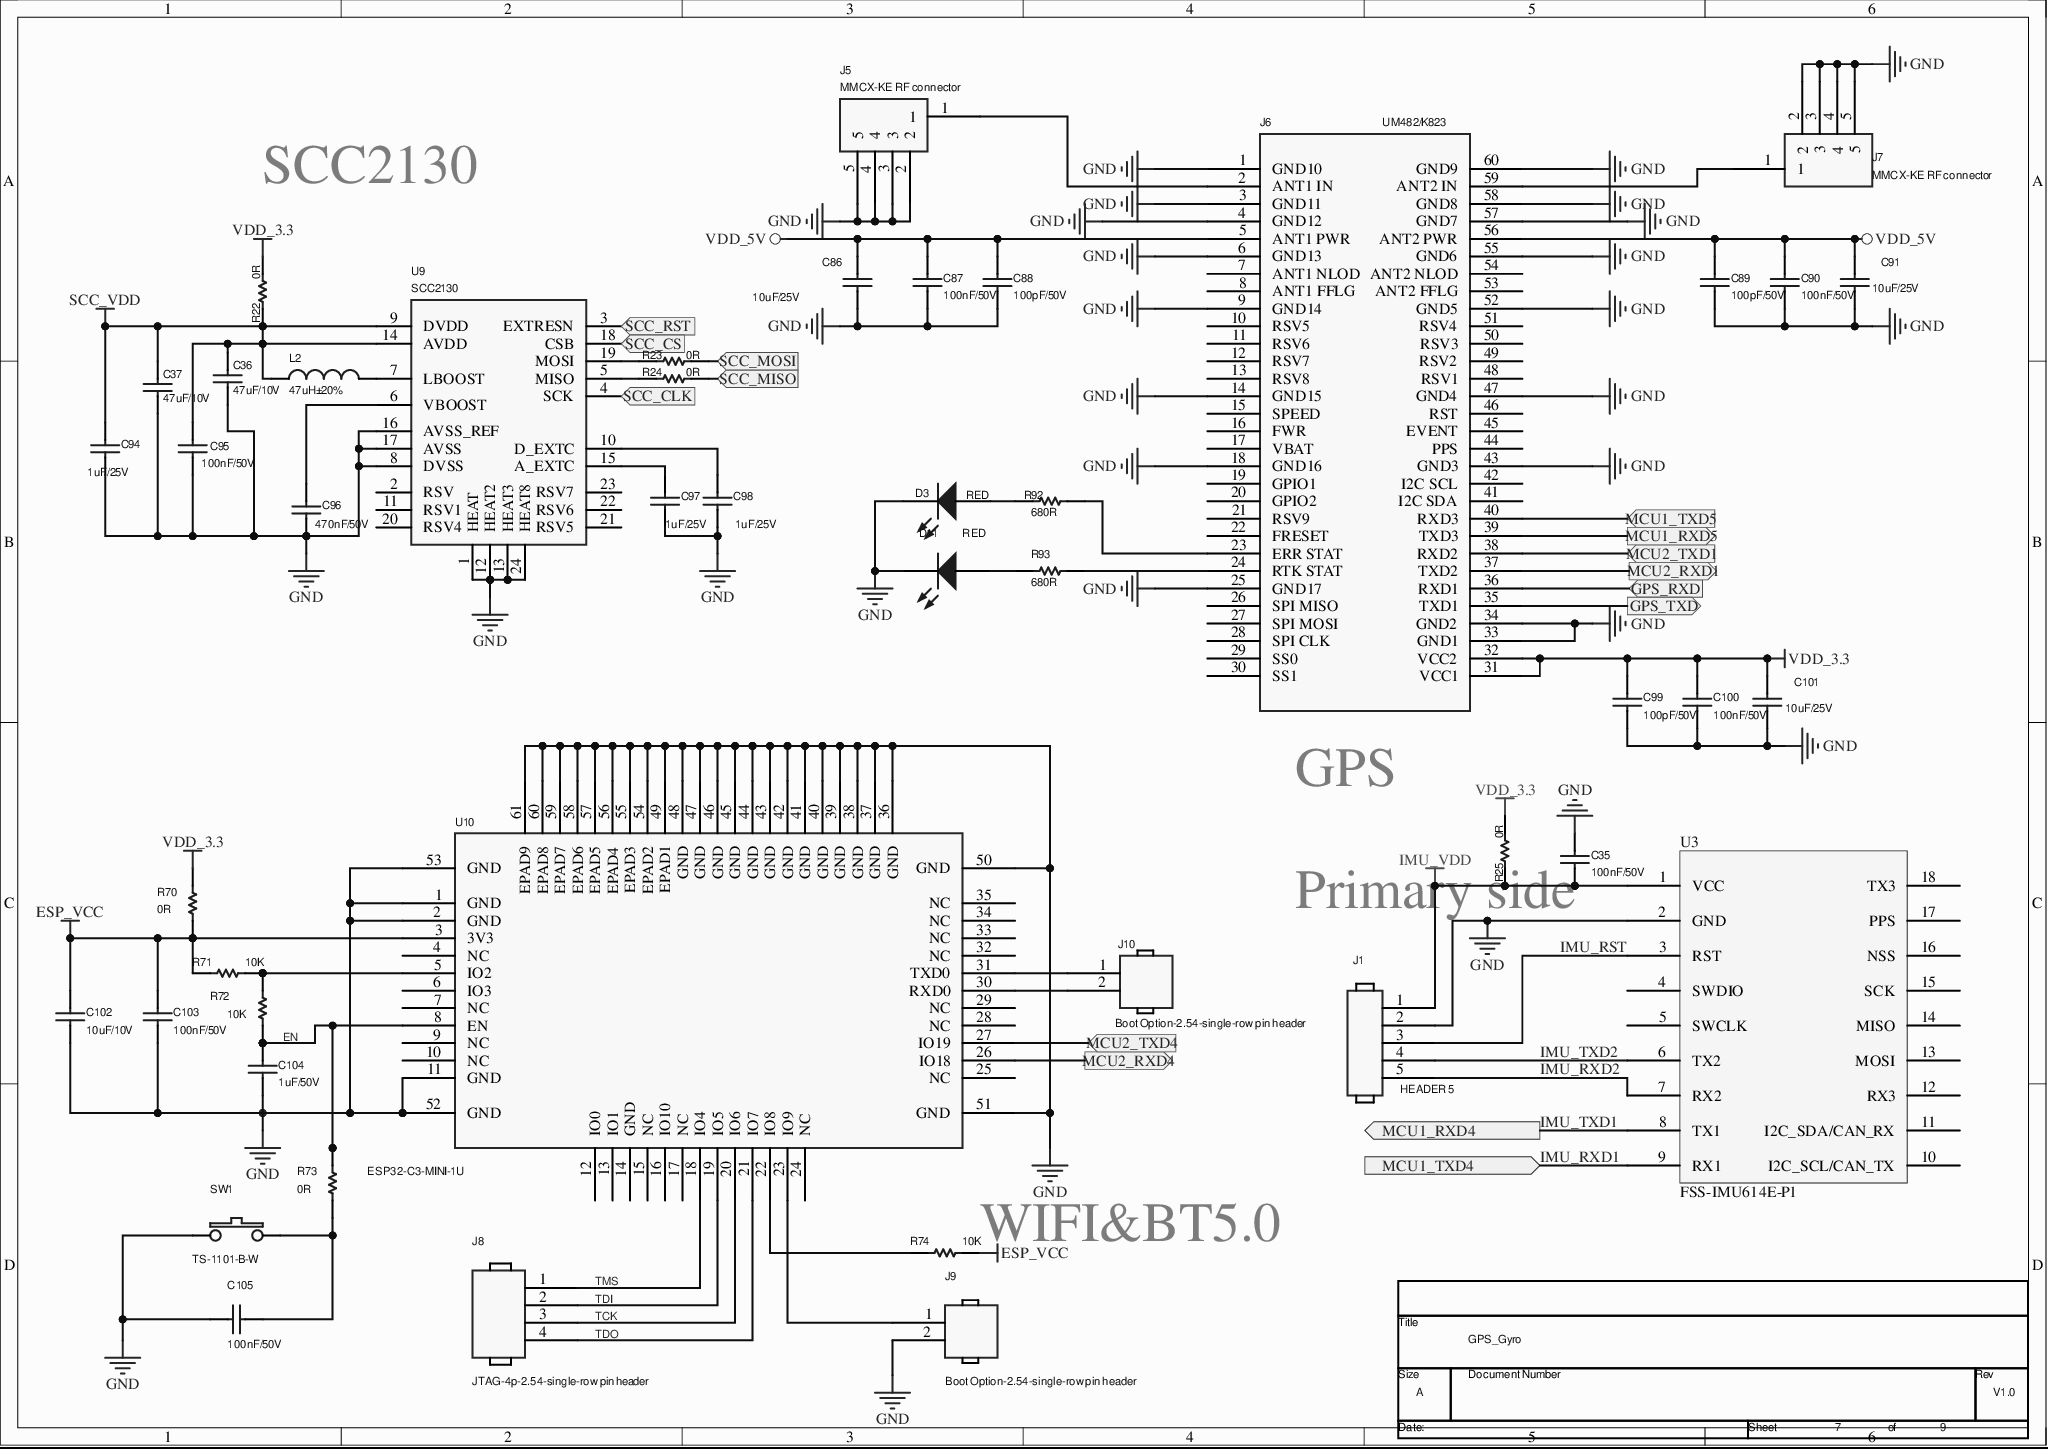
[diagram p0: MISC86294-14.SchDoc]
# Altium project MISC86294-22.PrjPcb (part 5 of 5)

## Sheet MISC86294-14.SchDoc
size 297 x 209 mm

### Parts
(Parts that share a designator on the sheet are numbered #1, #2 ... from top to bottom, then left to right.)
*#6  RevCode: V1.0  Title: GPS_Gyro  Page Size: A  Page Number: 7  Page Count: 9  (hidden comment: TitleBlock0)  (graphical)
C35  100nF/50V  [0603]
C36  47uF/10V  [CAP-SMD_L3.5-W2.8]
C37  47uF/10V  [CAP-SMD_L3.5-W2.8]
C86  10uF/25V  [C0805]
C87  100nF/50V  [0603]
C88  100pF/50V  [0603]
C89  100pF/50V  [0603]
C90  100nF/50V  [0603]
C91  10uF/25V  [C0805]
C94  1uF/25V  [0603]
C95  100nF/50V  [0603]
C96  470nF/50V  [0603]
C97  1uF/25V  [0603]
C98  1uF/25V  [0603]
C99  100pF/50V  [0603]
C100  100nF/50V  [0603]
C101  10uF/25V  [C0805]
C102  User_Value: 10uF/10V  [C0603]  (hidden comment: 100nF/50V)
C103  100nF/50V  [C0603]
C104  User_Value: 1uF/50V  [C0603]  (hidden comment: 100nF/50V)
C105  100nF/50V  [C0603]
D3  RED  [LED_0805]
D11  RED  [LED_0805]
J1  HEADER 5  [2.54mm_paizhen_5pin]
J5  MMCX-KE RF connector  [MMCX-KE]
J6  UM482/K823  [UM482_K823]
J7  MMCX-KE RF connector  [MMCX-KE]
J8  JTAG-4p-2.54-single-row pin header  [HDR_1X4_254]
J9  Boot Option-2.54-single-row pin header  [HDR_1X2_254]
J10  Boot Option-2.54-single-row pin header  [HDR_1X2_254]
L2  47uH±20%  [1210]
R22  0R  [R0603]
R23  0R  [R0603]
R24  0R  [R0603]
R25  0R  [R0603]
R70  0R  [R0603]
R71  10K  [R0603]
R72  10K  [R0603]
R73  0R  [R0603]
R74  10K  [R0603]
R92  User_Value: 680R  [0603]  (hidden comment: NA)
R93  User_Value: 680R  [0603]  (hidden comment: NA)
SW1  TS-1101-B-W  [SMD]
U3  FSS-IMU614E-P1  [FSS-IMU614E-P1]
U9  SCC2130  [SCC2130D]
U10  ESP32-C3-MINI-1U  [WIFIM-SMD_ESP32-C3-MINI-1]

### Ports
GPS_RXD (in), GPS_TXD (out), MCU1_RXD4 (out), MCU1_RXD5 (out), MCU1_TXD4 (in), MCU1_TXD5 (in), MCU2_RXD1 (out), MCU2_RXD4 (out), MCU2_TXD1 (in), MCU2_TXD4 (in), SCC_CLK (in), SCC_CS (in), SCC_MISO (in), SCC_MOSI (in), SCC_RST (in)

### Nets
ESP_VCC: C102.2 C103.2 R70.2 R71.2 R74.1 U10.3(3V3)
GND: C35.2 C36.2 C37.2 C86.1 C87.2 C88.2 C89.1 C90.1 C91.1 C94.2 C95.2 C96.2 C97.2 C98.2 C99.1 C100.1 C101.1 C102.1 C103.1 C104.1 C105.2 D3.2(K) D11.2(K) J1.2 J5.2 J5.3 J5.4 J5.5 J6.1(GND10) J6.3(GND11) J6.4(GND12) J6.6(GND13) J6.9(GND14) J6.14(GND15) J6.18(GND16) J6.25(GND17) J6.33(GND1) J6.34(GND2) J6.43(GND3) J6.47(GND4) J6.52(GND5) J6.55(GND6) J6.57(GND7) J6.58(GND8) J6.60(GND9) J7.2 J7.3 J7.4 J7.5 J9.2 SW1.1 U3.2(GND) U9.1(HEAT) U9.8(DVSS) U9.12(HEAT2) U9.13(HEAT3) U9.16(AVSS_REF) U9.17(AVSS) U9.24(HEAT8) U10.1(GND) U10.2(GND) U10.11(GND) U10.36(GND) U10.37(GND) U10.38(GND) U10.39(GND) U10.40(GND) U10.41(GND) U10.42(GND) U10.43(GND) U10.44(GND) U10.45(GND) U10.46(GND) U10.47(GND) U10.48(GND) U10.49(EPAD1) U10.50(GND) U10.51(GND) U10.52(GND) U10.53(GND) U10.54(EPAD2) U10.55(EPAD3) U10.56(EPAD4) U10.57(EPAD5) U10.58(EPAD6) U10.59(EPAD7) U10.60(EPAD8) U10.61(EPAD9)
IMU_VDD: C35.1 J1.1 R25.2 U3.1(VCC)
SCC_VDD: C36.1 C37.1 C94.1 C95.1 L2.1 R22.2 U9.9(DVDD) U9.14(AVDD)
VDD_3.3: C99.2 C100.2 C101.2 J6.31(VCC1) J6.32(VCC2) R22.1 R25.1 R70.1
VDD_5V: C86.2 C87.1 C88.1 C89.2 C90.2 C91.2 J6.5(ANT1_PWR) J6.56(ANT2_PWR)
EN: C104.2 R72.2 R73.1 U10.8(EN)
IMU_RST: J1.3 U3.3(RST)
IMU_RXD1: U3.9(RX1) ; port MCU1_TXD4
IMU_RXD2: J1.5 U3.7(RX2)
IMU_TXD1: U3.8(TX1) ; port MCU1_RXD4
IMU_TXD2: J1.4 U3.6(TX2)
TCK: J8.3 U10.20(IO6)
TDI: J8.2 U10.19(IO5)
TDO: J8.4 U10.21(IO7)
TMS: J8.1 U10.18(IO4)
NetC96_1: C96.1 U9.6(VBOOST)
NetC97_1: C97.1 U9.15(A_EXTC)
NetC98_1: C98.1 U9.10(D_EXTC)
NetC105_1: C105.1 R73.2 SW1.2
NetD3_1: D3.1(A) R92.2
NetD11_1: D11.1(A) R93.2
NetJ5_1: J5.1 J6.2(ANT1_IN)
NetJ6_23: J6.23(ERR_STAT) R92.1
NetJ6_24: J6.24(RTK_STAT) R93.1
NetJ6_35: J6.35(TXD1) ; port GPS_TXD
NetJ6_36: J6.36(RXD1) ; port GPS_RXD
NetJ6_37: J6.37(TXD2) ; port MCU2_RXD1
NetJ6_38: J6.38(RXD2) ; port MCU2_TXD1
NetJ6_39: J6.39(TXD3) ; port MCU1_RXD5
NetJ6_40: J6.40(RXD3) ; port MCU1_TXD5
NetJ6_59: J6.59(ANT2_IN) J7.1
NetJ9_1: J9.1 U10.23(IO9)
NetJ10_1: J10.1 U10.31(TXD0)
NetJ10_2: J10.2 U10.30(RXD0)
NetJ19_1: U10.27(IO19) ; port MCU2_TXD4
NetJ19_2: U10.26(IO18) ; port MCU2_RXD4
NetL2_2: L2.2 U9.7(LBOOST)
NetR23_1: R23.1 ; port SCC_MOSI
NetR23_2: R23.2 U9.19(MOSI)
NetR24_1: R24.1 ; port SCC_MISO
NetR24_2: R24.2 U9.5(MISO)
NetR71_1: R71.1 R72.1 U10.5(IO2)
NetR74_2: R74.2 U10.22(IO8)
NetU1_40: U9.18(CSB) ; port SCC_CS
NetU1_41: U9.4(SCK) ; port SCC_CLK
NetU1_44: U9.3(EXTRESN) ; port SCC_RST

Not connected (* = marked no-connect by the designer): J6 7(ANT1_NLOD) 8(ANT1_FFLG) 10(RSV5) 11(RSV6) 12(RSV7) 13(RSV8) 15(SPEED) 16(FWR) 17(VBAT) 19(GPIO1) 20(GPIO2) 21(RSV9) 22(FRESET) 26(SPI_MISO) 27(SPI_MOSI) 28(SPI_CLK) 29(SS0) 30(SS1) 41(I2C_SDA) 42(I2C_SCL) 44(PPS) 45(EVENT) 46(RST) 48(RSV1) 49(RSV2) 50(RSV3) 51(RSV4) 53(ANT2_FFLG) 54(ANT2_NLOD); U3 4(SWDIO) 5(SWCLK) 10(I2C_SCL/CAN_TX) 11(I2C_SDA/CAN_RX) 12(RX3) 13(MOSI) 14(MISO) 15(SCK) 16(NSS) 17(PPS) 18(TX3); U9 2(RSV) 11(RSV1) 20(RSV4) 21(RSV5) 22(RSV6) 23(RSV7); U10 4(NC) 6(IO3) 7(NC) 9(NC) 10(NC) 12(IO0) 13(IO1) 14(GND) 15(NC) 16(IO10) 17(NC) 24(NC) 25(NC) 28(NC) 29(NC) 32(NC) 33(NC) 34(NC) 35(NC)

### Notes on the sheet
- SCC2130
- (near J6) GPS
- Primary side
- (near R74) WIFI&BT5.0

### Library data of the parts
*#6 = TitleBlock0: Document: Agr-Ctrl-3GS-07; Page Create Date: March  8, 1995
C35 C100 = Cap_C17: Kind: General; SubKind: Capacitor; Origin: Altium; Published: 8-Jun-2000; LatestRevisionDate: 17-Jul-2002; LatestRevisionNote: Re-released for DXP Platform.; PackageReference: RAD-0.3; User_Value: 100nF/50V; Created: 1/08/1993; Spice Prefix: C; Type: Capacitor; Publisher: Altium Limited
C36 C37 = Cap_C2: Origin: Altium; Published: 8-Jun-2000; LatestRevisionDate: 17-Jul-2002; LatestRevisionNote: Re-released for DXP Platform.; PackageReference: RAD-0.3; User_Value: 47uF/10V; Created: 1/08/1993; Publisher: Altium Limited
C86 = Cap_C3: Kind: General; SubKind: Capacitor; Origin: Altium; Published: 8-Jun-2000; LatestRevisionDate: 17-Jul-2002; LatestRevisionNote: Re-released for DXP Platform.; PackageReference: RAD-0.3; User_Value: 10uF/25V; Created: 1/08/1993; Spice Prefix: C; Type: Capacitor; Publisher: Altium Limited
C87 = Cap_C5: Kind: General; SubKind: Capacitor; Origin: Altium; Published: 8-Jun-2000; LatestRevisionDate: 17-Jul-2002; LatestRevisionNote: Re-released for DXP Platform.; PackageReference: RAD-0.3; User_Value: 100nF/50V; Created: 1/08/1993; Spice Prefix: C; Type: Capacitor; Publisher: Altium Limited
C88 = Cap_C6: Kind: General; SubKind: Capacitor; Origin: Altium; Published: 8-Jun-2000; LatestRevisionDate: 17-Jul-2002; LatestRevisionNote: Re-released for DXP Platform.; PackageReference: RAD-0.3; User_Value: 100pF/50V; Created: 1/08/1993; Spice Prefix: C; Type: Capacitor; Publisher: Altium Limited
C89 = Cap_C7: Kind: General; SubKind: Capacitor; Origin: Altium; Published: 8-Jun-2000; LatestRevisionDate: 17-Jul-2002; LatestRevisionNote: Re-released for DXP Platform.; PackageReference: RAD-0.3; User_Value: 100pF/50V; Created: 1/08/1993; Spice Prefix: C; Type: Capacitor; Publisher: Altium Limited
C90 = Cap_C8: Kind: General; SubKind: Capacitor; Origin: Altium; Published: 8-Jun-2000; LatestRevisionDate: 17-Jul-2002; LatestRevisionNote: Re-released for DXP Platform.; PackageReference: RAD-0.3; User_Value: 100nF/50V; Created: 1/08/1993; Spice Prefix: C; Type: Capacitor; Publisher: Altium Limited
C91 = Cap_C4: Kind: General; SubKind: Capacitor; Origin: Altium; Published: 8-Jun-2000; LatestRevisionDate: 17-Jul-2002; LatestRevisionNote: Re-released for DXP Platform.; PackageReference: RAD-0.3; User_Value: 10uF/25V; Created: 1/08/1993; Spice Prefix: C; Type: Capacitor; Publisher: Altium Limited
C94 = Cap_C9: Kind: General; SubKind: Capacitor; Origin: Altium; Published: 8-Jun-2000; Revision: July-2002: Re-released for DXP Platform.; User_Value: 1uF/25V; Spice Prefix: C; Type: Capacitor; Publisher: Altium Limited
C95 = Cap_C10: Kind: General; SubKind: Capacitor; Origin: Altium; Published: 8-Jun-2000; Revision: July-2002: Re-released for DXP Platform.; User_Value: 100nF/50V; Spice Prefix: C; Type: Capacitor; Publisher: Altium Limited
C96 = Cap_C13: Kind: General; SubKind: Capacitor; Origin: Altium; Published: 8-Jun-2000; Revision: July-2002: Re-released for DXP Platform.; User_Value: 470nF/50V; Spice Prefix: C; Type: Capacitor; Publisher: Altium Limited
C97 = Cap_C11: Kind: General; SubKind: Capacitor; Origin: Altium; Published: 8-Jun-2000; Revision: July-2002: Re-released for DXP Platform.; User_Value: 1uF/25V; Spice Prefix: C; Type: Capacitor; Publisher: Altium Limited
C98 = Cap_C12: Kind: General; SubKind: Capacitor; Origin: Altium; Published: 8-Jun-2000; Revision: July-2002: Re-released for DXP Platform.; User_Value: 1uF/25V; Spice Prefix: C; Type: Capacitor; Publisher: Altium Limited
C99 = Cap_C16: Kind: General; SubKind: Capacitor; Origin: Altium; Published: 8-Jun-2000; LatestRevisionDate: 17-Jul-2002; LatestRevisionNote: Re-released for DXP Platform.; PackageReference: RAD-0.3; User_Value: 100pF/50V; Created: 1/08/1993; Spice Prefix: C; Type: Capacitor; Publisher: Altium Limited
C101 = Cap_C15: Kind: General; SubKind: Capacitor; Origin: Altium; Published: 8-Jun-2000; LatestRevisionDate: 17-Jul-2002; LatestRevisionNote: Re-released for DXP Platform.; PackageReference: RAD-0.3; User_Value: 10uF/25V; Created: 1/08/1993; Spice Prefix: C; Type: Capacitor; Publisher: Altium Limited
C102-C105 = Cap_C90: Kind: General; SubKind: Capacitor; Origin: Altium; Published: 8-Jun-2000; LatestRevisionDate: 17-Jul-2002; LatestRevisionNote: Re-released for DXP Platform.; PackageReference: RAD-0.3; Created: 1/08/1993; Spice Prefix: C; Type: Capacitor; Publisher: Altium Limited
  C103 C105: User_Value: 100nF/50V
D3 D11 = LED1_D4: Kind: General; SubKind: Diode; Origin: Altium; Published: 8-Jun-2000; LatestRevisionDate: 08-Jul-2005; LatestRevisionNote: Mech Layer 1 removed.; PackageReference: LED-1; Spice Prefix: D; Publisher: Altium Limited
J5 = CIRCLE_J1: Origin: Altium
J6 = UM482_J2: Origin: Altium
J7 = CIRCLE_J3: Origin: Altium
J8 = HEADER 4
J9 J10 = HEADER 2
L2 = Inductor_L1: Code_IEC: 1005; Origin: Altium; Published: 8-Jun-2000; LatestRevisionDate: 29-May-2009; LatestRevisionNote: IPC-7351 Footprint Added.; PackageReference: 0402-A; PackageDescription: Chip Inductor; Code_JEITA: 0402; User_Value: 47uH±20%; Created: 28/07/2004; Publisher: Altium Limited
R22-R25 R70-R74 = Res1_R57: Kind: General; SubKind: Resistor; Origin: Altium; Published: 8-Jun-2000; LatestRevisionDate: 17-Jul-2002; LatestRevisionNote: Re-released for DXP Platform.; PackageReference: AXIAL-0.3; Created: 1/08/1993; Spice Prefix: R; Type: Resistor; Publisher: Altium Limited
  R22-R25 R70 R73: User_Value: 0R
  R71 R72 R74: User_Value: 10K
R92 R93 = Res1_R8: Origin: Altium; Published: 8-Jun-2000; LatestRevisionDate: 17-Jul-2002; LatestRevisionNote: Re-released for DXP Platform.; PackageReference: AXIAL-0.3; Publisher: Altium Limited
SW1 = SW_PB_SPST
U3 = FSS-IMU614-AG
U9 = SCC2130_U2: Origin: Altium

## Sheet MISC86294-16.SchDoc
size 297 x 209 mm
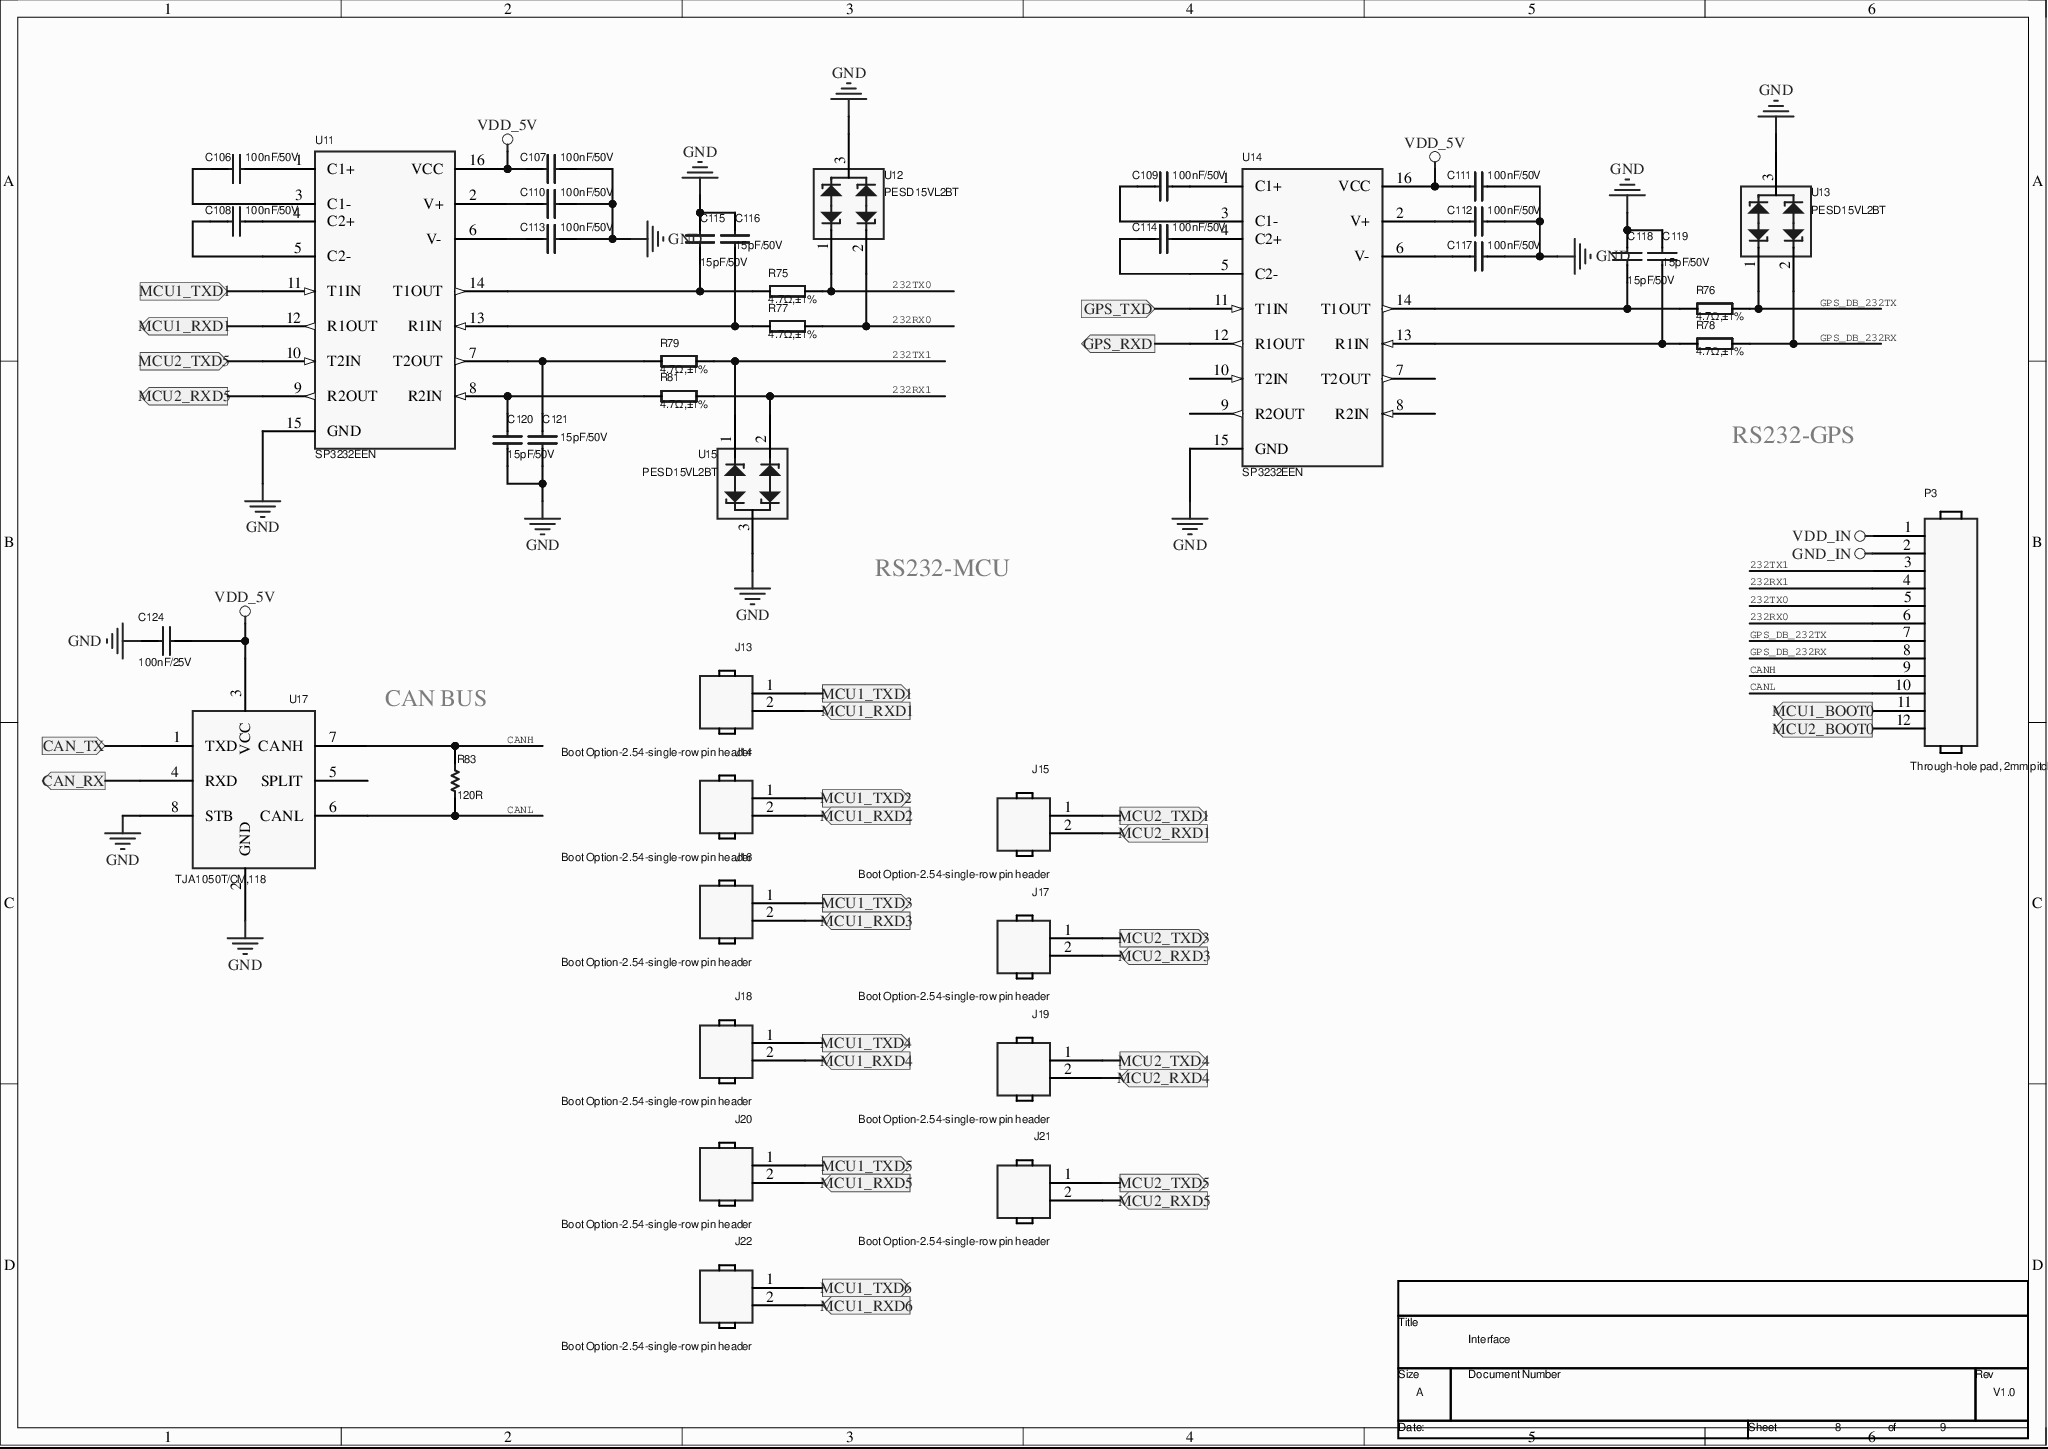
[diagram p1: MISC86294-16.SchDoc]

### Parts
(Parts that share a designator on the sheet are numbered #1, #2 ... from top to bottom, then left to right.)
*#7  RevCode: V1.0  Title: Interface  Page Size: A  Page Number: 8  Page Count: 9  (hidden comment: TitleBlock0)  (graphical)
C106  100nF/50V  [0603]
C107  100nF/50V  [0603]
C108  100nF/50V  [0603]
C109  100nF/50V  [0603]
C110  100nF/50V  [0603]
C111  100nF/50V  [0603]
C112  100nF/50V  [0603]
C113  100nF/50V  [0603]
C114  100nF/50V  [0603]
C115  15pF/50V  [0603]
C116  15pF/50V  [0603]
C117  100nF/50V  [0603]
C118  15pF/50V  [0603]
C119  15pF/50V  [0603]
C120  15pF/50V  [0603]
C121  15pF/50V  [0603]
C124  User_Value: 100nF/25V  [C0603]  (hidden comment: 100nF/50V)
J13  Boot Option-2.54-single-row pin header  [HDR_1X2_254]
J14  Boot Option-2.54-single-row pin header  [HDR_1X2_254]
J15  Boot Option-2.54-single-row pin header  [HDR_1X2_254]
J16  Boot Option-2.54-single-row pin header  [HDR_1X2_254]
J17  Boot Option-2.54-single-row pin header  [HDR_1X2_254]
J18  Boot Option-2.54-single-row pin header  [HDR_1X2_254]
J19  Boot Option-2.54-single-row pin header  [HDR_1X2_254]
J20  Boot Option-2.54-single-row pin header  [HDR_1X2_254]
J21  Boot Option-2.54-single-row pin header  [HDR_1X2_254]
J22  Boot Option-2.54-single-row pin header  [HDR_1X2_254]
P3  Through-hole pad, 2mm pitch  [XH-12A]
R75  4.7Ω,±1%  [0603]
R76  4.7Ω,±1%  [0603]
R77  4.7Ω,±1%  [0603]
R78  4.7Ω,±1%  [0603]
R79  4.7Ω,±1%  [0603]
R81  4.7Ω,±1%  [0603]
R83  120R  [R0603]
U11  SP3232EEN  [SOP16-6_6]
U12  PESD15VL2BT  [SOT-23]
U13  PESD15VL2BT  [SOT-23]
U14  SP3232EEN  [SOP16-6_6]
U15  PESD15VL2BT  [SOT-23]
U17  TJA1050T/CM,118  [SOIC-8]

### Ports
CAN_RX (out), CAN_TX (in), GPS_RXD (out), GPS_TXD (in), MCU1_BOOT0 (out), MCU1_RXD1 (in), MCU1_RXD1 (out), MCU1_RXD2 (in), MCU1_RXD3 (in), MCU1_RXD4 (in), MCU1_RXD5 (in), MCU1_RXD6 (in), MCU1_TXD1 (in), MCU1_TXD1 (out), MCU1_TXD2 (out), MCU1_TXD3 (out), MCU1_TXD4 (out), MCU1_TXD5 (out), MCU1_TXD6 (out), MCU2_BOOT0 (out), MCU2_RXD1 (in), MCU2_RXD3 (in), MCU2_RXD4 (in), MCU2_RXD5 (in), MCU2_RXD5 (out), MCU2_TXD1 (out), MCU2_TXD3 (out), MCU2_TXD4 (out), MCU2_TXD5 (in), MCU2_TXD5 (out)

### Nets
GND: C107.2 C110.2 C111.2 C112.2 C113.2 C115.1 C116.1 C117.2 C118.1 C119.1 C120.2 C121.2 C124.1 U11.15(GND) U12.3 U13.3 U14.15(GND) U15.3 U17.2(GND) U17.8(STB)
GND_IN: P3.2
VDD_5V: C107.1 C111.1 C124.2 U11.16(VCC) U14.16(VCC) U17.3(VCC)
VDD_IN: P3.1
232RX0: P3.6 R77.1 U12.2
232RX1: P3.4 R81.1 U15.2
232TX0: P3.5 R75.1 U12.1
232TX1: P3.3 R79.1 U15.1
CANH: P3.9 R83.1 U17.7(CANH)
CANL: P3.10 R83.2 U17.6(CANL)
GPS_DB_232RX: P3.8 R78.1 U13.2
GPS_DB_232TX: P3.7 R76.1 U13.1
IMU_RXD1: J18.1 ; port MCU1_TXD4
IMU_TXD1: J18.2 ; port MCU1_RXD4
NetC106_1: C106.1 U11.3(C1-)
NetC106_2: C106.2 U11.1(C1+)
NetC108_1: C108.1 U11.5(C2-)
NetC108_2: C108.2 U11.4(C2+)
NetC109_1: C109.1 U14.3(C1-)
NetC109_2: C109.2 U14.1(C1+)
NetC110_1: C110.1 U11.2(V+)
NetC112_1: C112.1 U14.2(V+)
NetC113_1: C113.1 U11.6(V-)
NetC114_1: C114.1 U14.5(C2-)
NetC114_2: C114.2 U14.4(C2+)
NetC115_2: C115.2 R75.2 U11.14(T1OUT)
NetC116_2: C116.2 R77.2 U11.13(R1IN)
NetC117_1: C117.1 U14.6(V-)
NetC118_2: C118.2 R76.2 U14.14(T1OUT)
NetC119_2: C119.2 R78.2 U14.13(R1IN)
NetC120_1: C120.1 R81.2 U11.8(R2IN)
NetC121_1: C121.1 R79.2 U11.7(T2OUT)
NetJ6_35: U14.11(T1IN) ; port GPS_TXD
NetJ6_36: U14.12(R1OUT) ; port GPS_RXD
NetJ6_37: J15.2 ; port MCU2_RXD1
NetJ6_38: J15.1 ; port MCU2_TXD1
NetJ6_39: J20.2 ; port MCU1_RXD5
NetJ6_40: J20.1 ; port MCU1_TXD5
NetJ13_1: J13.1 U11.11(T1IN) ; port MCU1_TXD1
NetJ13_2: J13.2 U11.12(R1OUT) ; port MCU1_RXD1
NetJ14_1: J14.1 ; port MCU1_TXD2
NetJ14_2: J14.2 ; port MCU1_RXD2
NetJ16_1: J16.1 ; port MCU1_TXD3
NetJ16_2: J16.2 ; port MCU1_RXD3
NetJ17_1: J17.1 ; port MCU2_TXD3
NetJ17_2: J17.2 ; port MCU2_RXD3
NetJ19_1: J19.1 ; port MCU2_TXD4
NetJ19_2: J19.2 ; port MCU2_RXD4
NetJ21_1: J21.1 U11.10(T2IN) ; port MCU2_TXD5
NetJ21_2: J21.2 U11.9(R2OUT) ; port MCU2_RXD5
NetJ22_1: J22.1 ; port MCU1_TXD6
NetJ22_2: J22.2 ; port MCU1_RXD6
NetP3_11: P3.11 ; port MCU1_BOOT0
NetP3_12: P3.12 ; port MCU2_BOOT0
NetU1_103: U17.4(RXD) ; port CAN_RX
NetU1_104: U17.1(TXD) ; port CAN_TX

Not connected (* = marked no-connect by the designer): U14 7(T2OUT) 8(R2IN) 9(R2OUT) 10(T2IN); U17 5(SPLIT)

### Notes on the sheet
- RS232-GPS
- RS232-MCU
- CAN BUS

### Library data of the parts
*#7 = TitleBlock0: Document: Agr-Ctrl-3GS-08; Page Create Date: March  8, 1995
C106 = Cap_C18: Origin: Altium; Published: 8-Jun-2000; Revision: July-2002: Re-released for DXP Platform.; User_Value: 100nF/50V; Publisher: Altium Limited
C107 = Cap_C19: Origin: Altium; Published: 8-Jun-2000; Revision: July-2002: Re-released for DXP Platform.; User_Value: 100nF/50V; Publisher: Altium Limited
C108 = Cap_C21: Origin: Altium; Published: 8-Jun-2000; Revision: July-2002: Re-released for DXP Platform.; User_Value: 100nF/50V; Publisher: Altium Limited
C109 = Cap_C36: Origin: Altium; Published: 8-Jun-2000; Revision: July-2002: Re-released for DXP Platform.; User_Value: 100nF/50V; Publisher: Altium Limited
C110 = Cap_C20: Origin: Altium; Published: 8-Jun-2000; Revision: July-2002: Re-released for DXP Platform.; User_Value: 100nF/50V; Publisher: Altium Limited
C111 = Cap_C37: Origin: Altium; Published: 8-Jun-2000; Revision: July-2002: Re-released for DXP Platform.; User_Value: 100nF/50V; Publisher: Altium Limited
C112 = Cap_C38: Origin: Altium; Published: 8-Jun-2000; Revision: July-2002: Re-released for DXP Platform.; User_Value: 100nF/50V; Publisher: Altium Limited
C113 = Cap_C24: Origin: Altium; Published: 8-Jun-2000; Revision: July-2002: Re-released for DXP Platform.; User_Value: 100nF/50V; Publisher: Altium Limited
C114 = Cap_C39: Origin: Altium; Published: 8-Jun-2000; Revision: July-2002: Re-released for DXP Platform.; User_Value: 100nF/50V; Publisher: Altium Limited
C115 = Cap_C22: Origin: Altium; Published: 8-Jun-2000; Revision: July-2002: Re-released for DXP Platform.; User_Value: 15pF/50V; Publisher: Altium Limited
C116 = Cap_C23: Origin: Altium; Published: 8-Jun-2000; Revision: July-2002: Re-released for DXP Platform.; User_Value: 15pF/50V; Publisher: Altium Limited
C117 = Cap_C42: Origin: Altium; Published: 8-Jun-2000; Revision: July-2002: Re-released for DXP Platform.; User_Value: 100nF/50V; Publisher: Altium Limited
C118 = Cap_C40: Origin: Altium; Published: 8-Jun-2000; Revision: July-2002: Re-released for DXP Platform.; User_Value: 15pF/50V; Publisher: Altium Limited
C119 = Cap_C41: Origin: Altium; Published: 8-Jun-2000; Revision: July-2002: Re-released for DXP Platform.; User_Value: 15pF/50V; Publisher: Altium Limited
C120 = Cap_C26: Origin: Altium; Published: 8-Jun-2000; Revision: July-2002: Re-released for DXP Platform.; User_Value: 15pF/50V; Publisher: Altium Limited
C121 = Cap_C27: Origin: Altium; Published: 8-Jun-2000; Revision: July-2002: Re-released for DXP Platform.; User_Value: 15pF/50V; Publisher: Altium Limited
C124 = Cap_C106: Kind: General; SubKind: Capacitor; Origin: Altium; Published: 8-Jun-2000; LatestRevisionDate: 17-Jul-2002; LatestRevisionNote: Re-released for DXP Platform.; PackageReference: RAD-0.3; Created: 1/08/1993; Spice Prefix: C; Type: Capacitor; Publisher: Altium Limited
J13-J22 = HEADER 2
P3 = HEADER 12
R75 = RES_R14: Origin: Altium; User_Value: 4.7Ω,±1%
R76 = RES_R22: Origin: Altium; User_Value: 4.7Ω,±1%
R77 = RES_R16: Origin: Altium; User_Value: 4.7Ω,±1%
R78 = RES_R23: Origin: Altium; User_Value: 4.7Ω,±1%
R79 = RES_R17: Origin: Altium; User_Value: 4.7Ω,±1%
R81 = RES_R18: Origin: Altium; User_Value: 4.7Ω,±1%
R83 = Res1_R90: Kind: General; SubKind: Resistor; Origin: Altium; Published: 8-Jun-2000; LatestRevisionDate: 17-Jul-2002; LatestRevisionNote: Re-released for DXP Platform.; PackageReference: AXIAL-0.3; User_Value: 120R; Created: 1/08/1993; Spice Prefix: R; Type: Resistor; Publisher: Altium Limited
U11 = SP202ECT_U3: Origin: Altium
U12 = PESD12VL2BT_U4: Origin: Altium
U13 = PESD12VL2BT_U8: Origin: Altium
U14 = SP202ECT_U7: Origin: Altium
U15 = PESD12VL2BT_U5: Origin: Altium
U17 = TJA1040T_U18: Origin: Altium

## Sheet MISC86294-18.SchDoc
size 297 x 209 mm
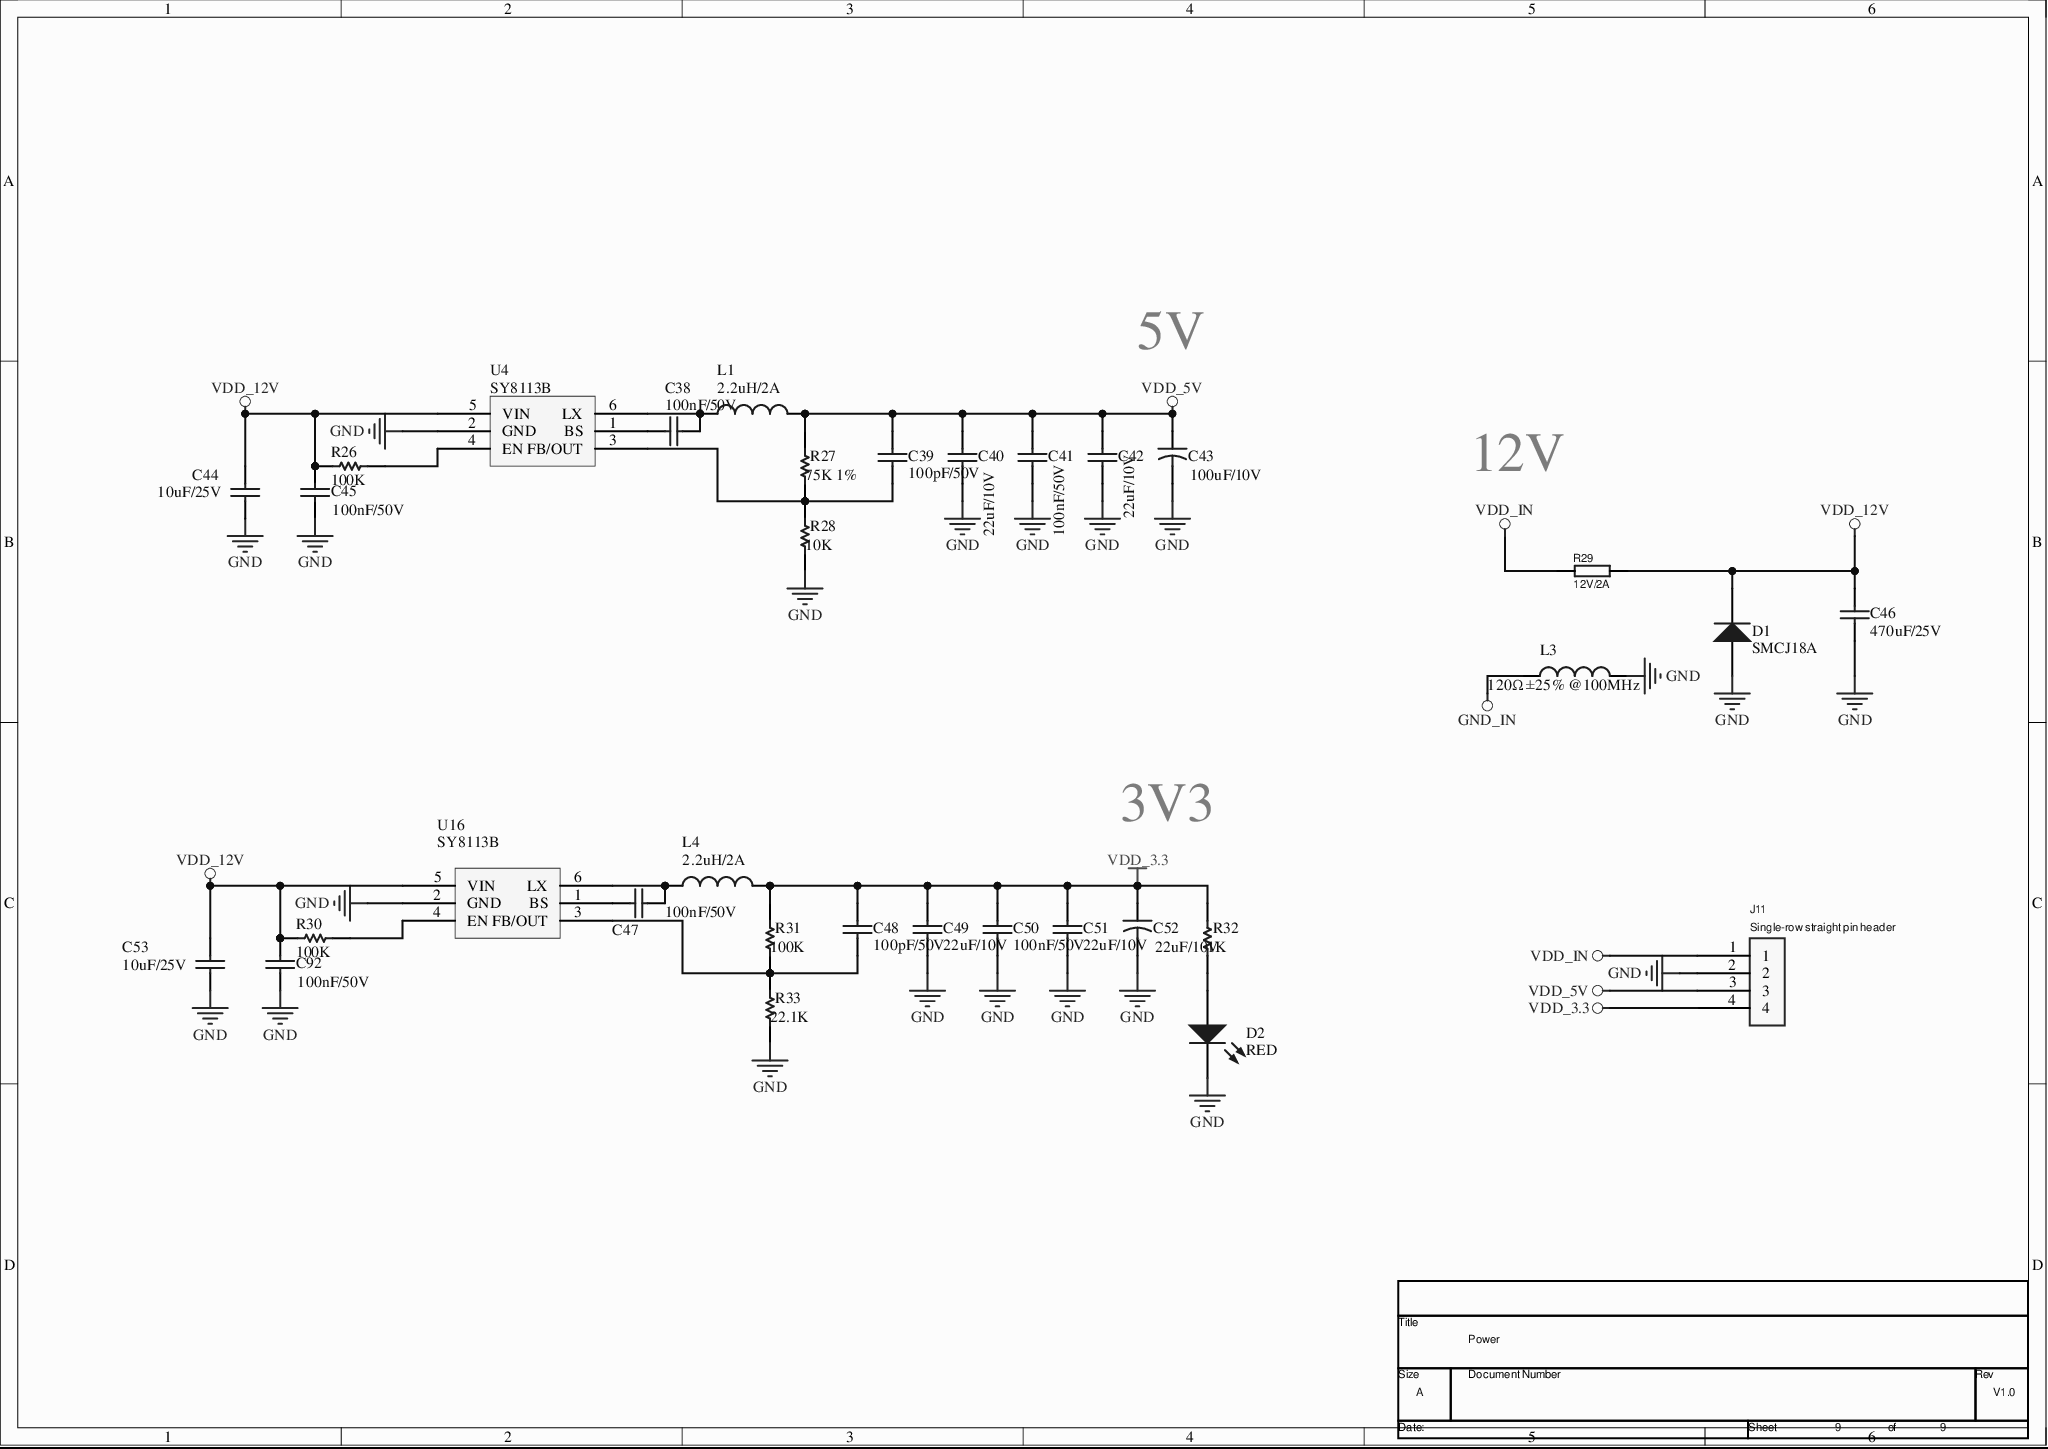
[diagram p2: MISC86294-18.SchDoc]

### Parts
(Parts that share a designator on the sheet are numbered #1, #2 ... from top to bottom, then left to right.)
*#8  RevCode: V1.0  Title: Power  Page Size: A  Page Number: 9  (hidden comment: TitleBlock0)  (graphical)
C38  100nF/50V  [0603]
C39  100pF/50V  [0603]
C40  22uF/10V  [C0805]
C41  100nF/50V  [0603]
C42  22uF/10V  [C0805]
C43  100uF/10V  [CAP-TH_BD5.0-P2.00-D0.8-FD]
C44  10uF/25V  [C0805]
C45  100nF/50V  [0603]
C46  470uF/25V  [CAP-TH_BD8.0-P3.50-D1.0-FD]
C47  100nF/50V  [0603]
C48  100pF/50V  [0603]
C49  22uF/10V  [C0805]
C50  100nF/50V  [0603]
C51  22uF/10V  [C0805]
C52  22uF/10V  [C0805]
C53  10uF/25V  [C0805]
C92  100nF/50V  [0603]
D1  SMCJ18A  [SMC_L6.9-W5.9-LS7.9-RD]
D2  RED  [LED_0805]
J11  Single-row straight pin header  [HDR1X4]
L1  2.2uH/2A  [IND-SMD_L4.0-W4.0]
L3  120Ω ±25% @100MHz  [0603]
L4  2.2uH/2A  [IND-SMD_L4.0-W4.0]
R26  100K  [0603]
R27  75K 1%  [0603]
R28  10K  [0603]
R29  12V/2A  [1210]
R30  100K  [0603]
R31  100K  [0603]
R32  1K  [0603]
R33  22.1K  [0603]
U4  SY8113B  [TSOT-23-6_L2.9-W1.6-P0.95-LS2.8-BR]
U16  SY8113B  [TSOT-23-6_L2.9-W1.6-P0.95-LS2.8-BR]

### Nets
GND: C40.2 C41.2 C42.2 C43.2 C44.1 C45.1 C46.2 C49.2 C50.2 C51.2 C52.2 C53.1 C92.1 D1.1(A) D2.2(K) J11.2 L3.2 R28.1 R33.1 U4.2(GND) U16.2(GND)
GND_IN: L3.1
VDD_3.3: C48.1 C49.1 C50.1 C51.1 C52.1 J11.4 L4.2 R31.2 R32.2
VDD_5V: C39.1 C40.1 C41.1 C42.1 C43.1 J11.3 L1.2 R27.2
VDD_12V: C44.2 C45.2 C46.1 C53.2 C92.2 D1.2(K) R26.2 R29.1 R30.2 U4.5(VIN) U16.5(VIN)
VDD_IN: J11.1 R29.2
NetC38_1: C38.1 L1.1 U4.6(LX)
NetC38_2: C38.2 U4.1(BS)
NetC39_2: C39.2 R27.1 R28.2 U4.3(FB/OUT)
NetC47_1: C47.1 L4.1 U16.6(LX)
NetC47_2: C47.2 U16.1(BS)
NetC48_2: C48.2 R31.1 R33.2 U16.3(FB/OUT)
NetD2_1: D2.1(A) R32.1
NetR26_1: R26.1 U4.4(EN)
NetR30_1: R30.1 U16.4(EN)

### Notes on the sheet
- 5V
- 12V
- 3V3

### Library data of the parts
*#8 = TitleBlock0: Document: Agr-Ctrl-3GS-09; Page Create Date: March  8, 1995; Page Count: 9
C38 C39 C41 C45 = Cap: SMD ceramic capacitor; Published: 8-Jun-2000; LatestRevisionDate: 17-Jul-2002; LatestRevisionNote: Re-released for DXP Platform.; PackageReference: RAD-0.3; Publisher: Altium Limited
  C38 C41 C45: Value: 100nF/50V
  C39: Value: 100pF/50V
C40 C42 = Cap: SMD ceramic capacitor, X5R; Published: 8-Jun-2000; LatestRevisionDate: 17-Jul-2002; LatestRevisionNote: Re-released for DXP Platform.; PackageReference: RAD-0.3; Value: 22uF/10V; Publisher: Altium Limited
C43 = Cap2: 100μF,10V,Φ5×7mm,RoHS; Published: 23-Sep-2002; PackageReference: CAPR5-4X5; Value: 100uF/10V; Publisher: Altium Limited
C44 = Cap: SMD ceramic capacitor, MLCC; Published: 8-Jun-2000; LatestRevisionDate: 17-Jul-2002; LatestRevisionNote: Re-released for DXP Platform.; PackageReference: RAD-0.3; Value: 10uF/25V; Publisher: Altium Limited
C46 = Cap: 470μF,25V,Φ8×11.5mm,RoHS; Published: 8-Jun-2000; LatestRevisionDate: 17-Jul-2002; LatestRevisionNote: Re-released for DXP Platform.; PackageReference: RAD-0.3; Value: 470uF/25V; Publisher: Altium Limited
C47-C51 C53 C92 = Cap: Capacitor; Published: 8-Jun-2000; LatestRevisionDate: 17-Jul-2002; LatestRevisionNote: Re-released for DXP Platform.; PackageReference: RAD-0.3; Publisher: Altium Limited
  C47 C50 C92: Value: 100nF/50V
  C48: Value: 100pF/50V
  C49 C51: Value: 22uF/10V
  C53: Value: 10uF/25V
C52 = Cap2: Capacitor; Published: 23-Sep-2002; PackageReference: CAPR5-4X5; Value: 22uF/10V; Publisher: Altium Limited
D1 = Diode: TVS diode; Published: 8-Jun-2000; LatestRevisionDate: 17-Jul-2002; LatestRevisionNote: Re-released for DXP Platform.; PackageVersion: Sep-1996; PackageReference: SMC; Code_JEDEC: DO-214-AB; Publisher: Altium Limited
D2 = LED1: Red high-brightness LED; Published: 8-Jun-2000; LatestRevisionDate: 08-Jul-2005; LatestRevisionNote: Mech Layer 1 removed.; PackageReference: LED-1; Publisher: Altium Limited
J11 = 2.54_J4: Origin: Altium; Application_BuildNumber: *
L1 L4 = Inductor: SMD power inductor, cjiang (Changjiang Micro), FNR4026S2R2MT; Code_IEC: 1005; Published: 8-Jun-2000; LatestRevisionDate: 29-May-2009; LatestRevisionNote: IPC-7351 Footprint Added.; PackageReference: 0402-A; PackageDescription: Chip Inductor; Code_JEITA: 0402; Value: 2.2uH/2A; Publisher: Altium Limited
L3 = Inductor: Ferrite bead; Code_IEC: 1005; Published: 8-Jun-2000; LatestRevisionDate: 29-May-2009; LatestRevisionNote: IPC-7351 Footprint Added.; PackageReference: 0402-A; PackageDescription: Chip Inductor; Code_JEITA: 0402; Publisher: Altium Limited
R26-R28 R30-R33 = Res1: SMD resistor; Published: 8-Jun-2000; LatestRevisionDate: 17-Jul-2002; LatestRevisionNote: Re-released for DXP Platform.; PackageReference: AXIAL-0.3; Publisher: Altium Limited
  R26 R30 R31: Value: 100K
  R27: Value: 75K 1%
  R28: Value: 10K
  R32: Value: 1K
  R33: Value: 22.1K
R29 = RES: Resettable fuse

## Nets that join several sheets
GND: MISC86294-6 (35 pins), MISC86294-8 (36 pins), MISC86294-12 (107 pins), MISC86294-14 (88 pins), MISC86294-16 (20 pins), MISC86294-18 (21 pins)
GND_IN: MISC86294-16 (P3.2), MISC86294-18 (L3.1)
VDD_3.3: MISC86294-6 (6 pins), MISC86294-8 (L201.2 R19.1 R84.1), MISC86294-12 (6 pins), MISC86294-14 (8 pins), MISC86294-18 (9 pins)
VDD_5V: MISC86294-12 (6 pins), MISC86294-14 (8 pins), MISC86294-16 (6 pins), MISC86294-18 (8 pins)
VDD_IN: MISC86294-16 (P3.1), MISC86294-18 (J11.1 R29.2)
IMU_RXD1: MISC86294-6 (U1.111), MISC86294-14 (U3.9), MISC86294-16 (J18.1)
IMU_TXD1: MISC86294-6 (U1.112), MISC86294-14 (U3.8), MISC86294-16 (J18.2)
NetJ6_35: MISC86294-14 (J6.35), MISC86294-16 (U14.11)
NetJ6_36: MISC86294-14 (J6.36), MISC86294-16 (U14.12)
NetJ6_37: MISC86294-8 (U2.102), MISC86294-14 (J6.37), MISC86294-16 (J15.2)
NetJ6_38: MISC86294-8 (U2.101), MISC86294-14 (J6.38), MISC86294-16 (J15.1)
NetJ6_39: MISC86294-6 (U1.116), MISC86294-14 (J6.39), MISC86294-16 (J20.2)
NetJ6_40: MISC86294-6 (U1.113), MISC86294-14 (J6.40), MISC86294-16 (J20.1)
NetJ13_1: MISC86294-6 (U1.101), MISC86294-16 (J13.1 U11.11)
NetJ13_2: MISC86294-6 (U1.102), MISC86294-16 (J13.2 U11.12)
NetJ14_1: MISC86294-6 (U1.36), MISC86294-8 (U2.37), MISC86294-16 (J14.1)
NetJ14_2: MISC86294-6 (U1.37), MISC86294-8 (U2.36), MISC86294-16 (J14.2)
NetJ16_1: MISC86294-6 (U1.69), MISC86294-16 (J16.1)
NetJ16_2: MISC86294-6 (U1.70), MISC86294-16 (J16.2)
NetJ17_1: MISC86294-8 (U2.69), MISC86294-12 (Q4.1), MISC86294-16 (J17.1)
NetJ17_2: MISC86294-8 (U2.70), MISC86294-12 (Q7.3 R44.1), MISC86294-16 (J17.2)
NetJ19_1: MISC86294-8 (U2.111), MISC86294-14 (U10.27), MISC86294-16 (J19.1)
NetJ19_2: MISC86294-8 (U2.112), MISC86294-14 (U10.26), MISC86294-16 (J19.2)
NetJ21_1: MISC86294-8 (U2.113), MISC86294-16 (J21.1 U11.10)
NetJ21_2: MISC86294-8 (U2.116), MISC86294-16 (J21.2 U11.9)
NetJ22_1: MISC86294-6 (U1.96), MISC86294-16 (J22.1)
NetJ22_2: MISC86294-6 (U1.97), MISC86294-16 (J22.2)
NetJ23_1: MISC86294-8 (U2.45), MISC86294-12 (J23.1 R91.1 U20.2)
NetP3_11: MISC86294-6 (R1.1 R2.2), MISC86294-16 (P3.11)
NetP3_12: MISC86294-8 (R13.1 R14.2), MISC86294-16 (P3.12)
NetQ3_1: MISC86294-8 (U2.74), MISC86294-12 (Q3.1)
NetQ5_1: MISC86294-8 (U2.79), MISC86294-12 (Q5.1)
NetQ6_3: MISC86294-8 (U2.75), MISC86294-12 (Q6.3 R42.1)
NetQ8_3: MISC86294-8 (U2.77), MISC86294-12 (Q8.3 R52.1)
NetQ9_3: MISC86294-8 (U2.78), MISC86294-12 (Q9.3 R55.1)
NetQ10_1: MISC86294-8 (U2.99), MISC86294-12 (Q10.1)
NetQ11_1: MISC86294-8 (U2.93), MISC86294-12 (Q11.1)
NetQ12_1: MISC86294-8 (U2.96), MISC86294-12 (Q12.1)
NetQ13_1: MISC86294-8 (U2.92), MISC86294-12 (Q13.1)
NetQ14_1: MISC86294-8 (U2.97), MISC86294-12 (Q14.1)
NetQ17_1: MISC86294-8 (U2.98), MISC86294-12 (Q17.1)
NetR23_1: MISC86294-6 (U1.43), MISC86294-14 (R23.1)
NetR24_1: MISC86294-6 (U1.42), MISC86294-14 (R24.1)
NetU1_34: MISC86294-6 (U1.34), MISC86294-8 (U2.35)
NetU1_35: MISC86294-6 (U1.35), MISC86294-8 (U2.34)
NetU1_40: MISC86294-6 (U1.40), MISC86294-14 (U9.18)
NetU1_41: MISC86294-6 (U1.41), MISC86294-14 (U9.4)
NetU1_44: MISC86294-6 (U1.44), MISC86294-14 (U9.3)
NetU1_103: MISC86294-6 (U1.103), MISC86294-16 (U17.4)
NetU1_104: MISC86294-6 (U1.104), MISC86294-16 (U17.1)